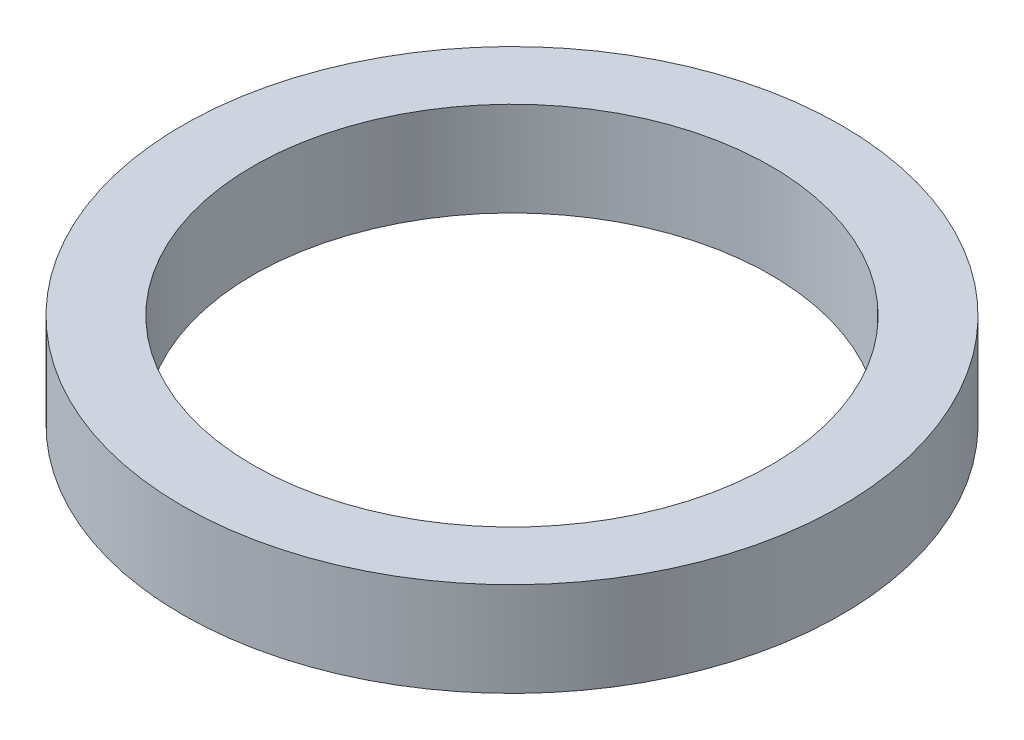
from build123d import *

# Parameters (mm, degrees)
SKETCH1_R           = 7
SKETCH1_R_2         = 5.5
BOSS_EXTRUDE1_DEPTH = 1


with BuildPart() as part:
    # Sketch1 → Boss-Extrude1 (new, symmetric)
    with BuildSketch(Plane(origin=(0, 0, 0), x_dir=(1, 0, 0), z_dir=(0, 1, 0))):
        with Locations(Location((0, 0, 0), (0, 0, 270))):
            Circle(SKETCH1_R)
        with Locations(Location((0, 0, 0), (0, 0, 270))):
            Circle(SKETCH1_R_2, mode=Mode.SUBTRACT)
    extrude(amount=BOSS_EXTRUDE1_DEPTH, both=True)


solid = part.part
